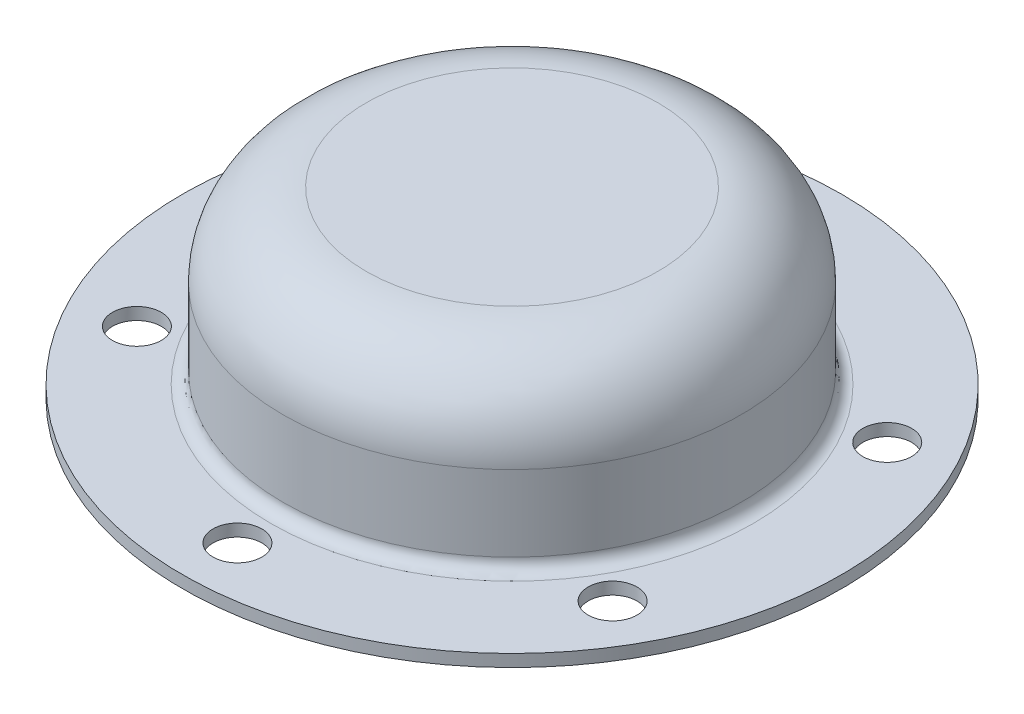
from build123d import *

# Parameters (mm, degrees)
SKETCH_2_R          = 4
CUT_EXTRUDE_1_DEPTH = 10


with BuildPart() as part:
    # 草图1 → 旋转1 (revolve)
    with BuildSketch(Plane.XY, mode=Mode.PRIVATE) as revolve_1_sk:
        with BuildLine():
            Line((54, -13), (39.5, -13))
            ThreePointArc((39.5, -13), (38.085786438, -12.414213562), (37.5, -11))
            Line((37.5, -11), (37.5, 1.42282291))
            ThreePointArc((37.5, 1.42282291), (33.5233369, 11.0233369), (23.92282291, 15))
            Line((23.92282291, 15), (0, 15))
            Line((0, 15), (0, 13))
            Line((0, 13), (23.92282291, 13))
            ThreePointArc((23.92282291, 13), (32.109123337, 9.609123337), (35.5, 1.42282291))
            Line((35.5, 1.42282291), (35.5, -13))
            ThreePointArc((35.5, -13), (36.085786438, -14.414213562), (37.5, -15))
            Line((37.5, -15), (54, -15))
            Line((54, -15), (54, -13))
        make_face()
    revolve(revolve_1_sk.sketch.rotate(Axis((0, 0, 0), (0, 1, 0)), 90), axis=Axis((0, 0, 0), (0, 1, 0)))

    # 草图2 → 切除-拉伸1 (cut)
    with BuildSketch(Plane(origin=(0, -13, 0), x_dir=(1, 0, 0), z_dir=(0, 1, 0))):
        with Locations(Location((0, 45, 0), (0, 0, 270))):
            Circle(SKETCH_2_R)
        with Locations(Location((38.97114317, 22.5, 0), (0, 0, 270))):
            Circle(SKETCH_2_R)
        with Locations(Location((38.97114317, -22.5, 0), (0, 0, 270))):
            Circle(SKETCH_2_R)
        with Locations(Location((0, -45, 0), (0, 0, 270))):
            Circle(SKETCH_2_R)
        with Locations(Location((-38.97114317, -22.5, 0), (0, 0, 270))):
            Circle(SKETCH_2_R)
        with Locations(Location((-38.97114317, 22.5, 0), (0, 0, 270))):
            Circle(SKETCH_2_R)
    extrude(amount=-CUT_EXTRUDE_1_DEPTH, mode=Mode.SUBTRACT)


solid = part.part
